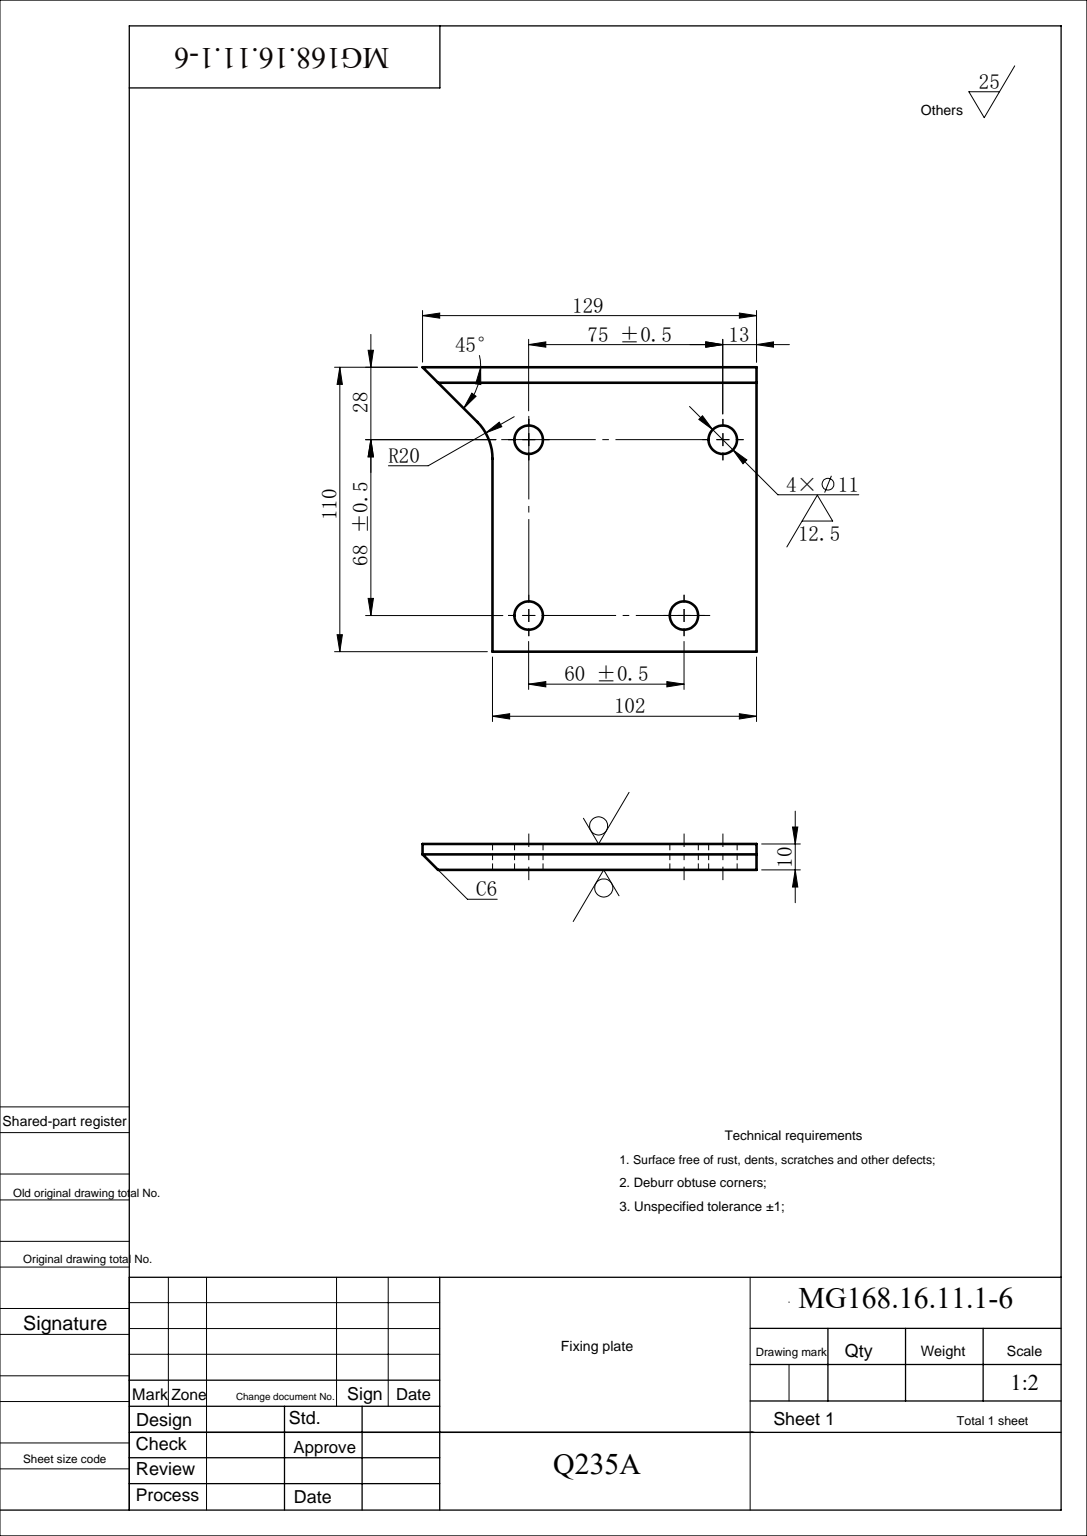
SolidWorks part; units mm, degrees
material "Q235A"
ref_plane "Front Plane" through (0, 0, 0) normal (0, 0, 1) x (1, 0, 0)
ref_plane "Top Plane" through (0, 0, 0) normal (0, 1, 0) x (1, 0, 0)
ref_plane "Right Plane" through (0, 0, 0) normal (1, 0, 0) x (0, 0, -1)
sketch "Sketch1" plane through (0, 0, 0) normal (0, 0, 1) x (1, 0, 0)
  line L0 (-65.1767, 0) -> (78.1015, 0) construction
  line L1 (-58, 96) -> (71, 96)
  line L2 (-58, 96) -> (-58, -14)
  line L3 (-58, -14) -> (44, -14)
  line L5 (50, 0) -> (-50, 0) construction
  line L6 (71, 96) -> (49.8579, 74.8579)
  line L7 (44, 60.7157) -> (44, -14)
  arc A0 (44, 60.7157) -> (49.8579, 74.8579) centre (64, 60.7157) cw
  point P13 (44, 69)
  dimension "D7" = 20
  dimension "D1" = 58
  dimension "D2" = 71
  dimension "D3" = 110
  dimension "D4" = 14
  dimension "D5" = 44
  dimension "D6" = 135
extrude "Boss-Extrude1" add sketch "Sketch1" along normal mid plane 10
sketch "Sketch2" plane through (0, 0, 0) normal (0, 0, 1) x (1, 0, 0)
  line L0 (50, 0) -> (-50, 0) construction
  line L1 (-66.9139, 68) -> (78.436, 68) construction
  line L2 (30, 105.6895) -> (30, -24.3497) construction
  circle A0 centre (-30, 0) radius 5.5
  circle A1 centre (30, 0) radius 5.5
  circle A2 centre (-45, 68) radius 5.5
  circle A3 centre (30, 68) radius 5.5
  dimension "D1" = 11
  dimension "D2" = 68
  dimension "D3" = 60
  dimension "D4" = 75
  dimension "D5" = 30
extrude "Cut-Extrude1" cut sketch "Sketch2" against normal through all both and the other way through all
chamfer "Chamfer1" distance 6 angle 45 1 edges at (6.5, 96, -5)
